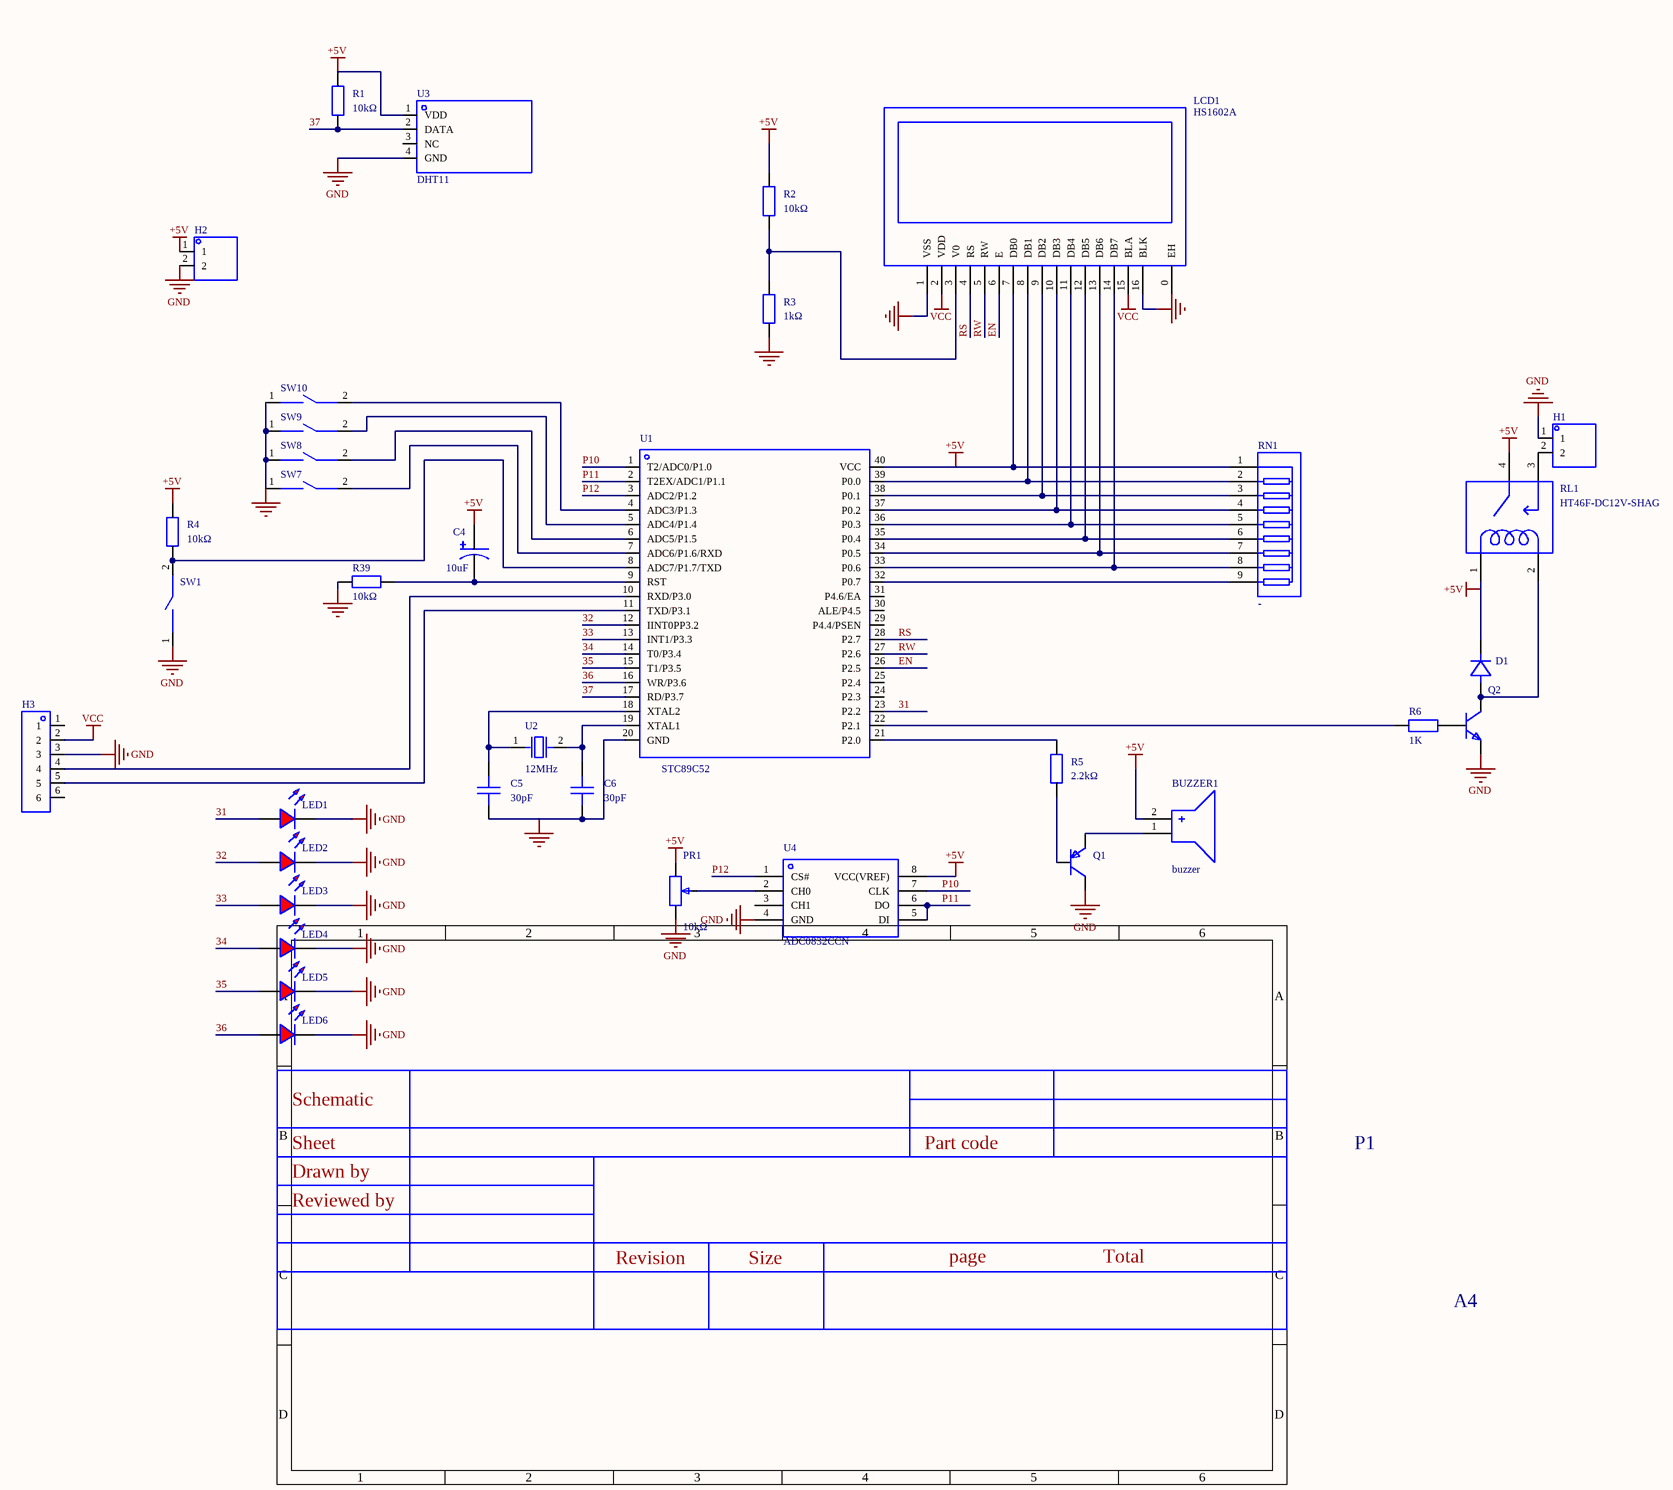
[diagram p0: MISC89128-3.schdoc]
# Altium project MISC89128-2.PrjPcb
1 sheet, 36 parts. Net scope: global (net labels, ports and power ports of the same name join across sheets).
Board file: MISC89128.pcbdoc

## Sheet MISC89128-3.schdoc
size 178 x 98 mm; Version: V1.0; @Project Name: MISC89128; @Page Count: 1; @Update Date: 2026-04-20; @Create Date: 2026-04-20; @Schematic Name: MISC89128; @Page No: 1; @Board Name: MISC89128; @Create Time: 15:46:19; @Update Time: 15:42:54

### Parts
BUZZER1  buzzer  [BUZ-TH_BD12.0-P6.00-D0.9-RD]
C4  10uF  [CAP-TH_BD6.3-P2.50-D1.0-FD]
C5  30pF  [CAP-TH_L3.6-W2.3-P5.00-D0.5]
C6  30pF  [CAP-TH_L3.6-W2.3-P5.00-D0.5]
D1  (no value)  [DO_1N4007]
H1  (no value)  [HDR-TH_2P-P2.54-V-M-1]
H2  (no value)  [HDR-TH_2P-P2.54-V-M-1]
H3  (no value)  [HDR-TH_6P-P2.54-V-F]
LCD1  HS1602A  [LCD1602]
LED1  (no value)  [LED_TH-3mm]
LED2  (no value)  [LED_TH-3mm]
LED3  (no value)  [LED_TH-3mm]
LED4  (no value)  [LED_TH-3mm]
LED5  (no value)  [LED_TH-3mm]
LED6  (no value)  [LED_TH-3mm]
PR1  10kΩ  [R_3296]
Q1  (no value)  [S8550P_SOT]
Q2  (no value)  [S8050_SOT-23]
R1  10kΩ  [Res_1/8W]
R2  10kΩ  [Res_1/8W]
R3  1kΩ  [Res_1/8W]
R4  10kΩ  [Res_1/8W]
R5  2.2kΩ  [Res_1/8W]
R6  1K  [R0805]
R39  10kΩ  [Res_1/8W]
RL1  HT46F-DC12V-SHAG  [RELAY-TH_HT46F-DCXXV-SHAG]
RN1  -  [RES-ARRAY-TH_9P-P2.54-D1.0]
SW1  Tact switch, 6*6*5 plastic head, 260G, travel 0.25mm, through-hole 2-pin  [KEY-TH_2P-L6.0-W6.0-P5.00]  (value not drawn)
SW7  Tact switch, 6*6*5 plastic head, 260G, travel 0.25mm, through-hole 2-pin  [KEY-TH_2P-L6.0-W6.0-P5.00]  (value not drawn)
SW8  Tact switch, 6*6*5 plastic head, 260G, travel 0.25mm, through-hole 2-pin  [KEY-TH_2P-L6.0-W6.0-P5.00]  (value not drawn)
SW9  Tact switch, 6*6*5 plastic head, 260G, travel 0.25mm, through-hole 2-pin  [KEY-TH_2P-L6.0-W6.0-P5.00]  (value not drawn)
SW10  Tact switch, 6*6*5 plastic head, 260G, travel 0.25mm, through-hole 2-pin  [KEY-TH_2P-L6.0-W6.0-P5.00]  (value not drawn)
U1  STC89C52  [DIP-40_L52.3-W13.9-P2.54-LS15.2-BL]
U2  12MHz  [HC-49US_L11.0-W4.6-P4.88]
U3  DHT11  [SENSOR-TH_DHT11]
U4  ADC0832CCN  [DIP-8_L9.7-W6.4-P2.54-LS7.6-BL]

### Nets
+5V: BUZZER1.2(+) C4.1 D1.1(K) H2.1 LCD1.7(DB0) PR1.3 R1.2 R2.2 R4.2 RL1.1 RL1.4 RN1.1 U1.40(VCC) U3.1(VDD) U4.8(VCC(VREF))
GND: C5.1 C6.1 H1.1 H2.2 H3.3 LCD1.1(VSS) LCD1.16(BLK) LED1.2(A) LED2.2(A) LED3.2(A) LED4.2(A) LED5.2(A) LED6.2(A) PR1.1 Q1.3(C) Q2.2 R3.1 R39.1 SW1.1 SW7.1 SW8.1 SW9.1 SW10.1 U1.20(GND) U3.4(GND) U4.4(GND)
VCC: H3.2 LCD1.2(VDD) LCD1.15(BLA)
31: LED1.1(C) U1.23(P2.2)
32: LED2.1(C) U1.12(IINT0PP3.2)
33: LED3.1(C) U1.13(INT1/P3.3)
34: LED4.1(C) U1.14(T0/P3.4)
35: LED5.1(C) U1.15(T1/P3.5)
36: LED6.1(C) U1.16(WR/P3.6)
37: R1.1 U1.17(RD/P3.7) U3.2(DATA)
EN: LCD1.6(E) U1.26(P2.5)
P10: U1.1(T2/ADC0/P1.0) U4.7(CLK)
P11: U1.2(T2EX/ADC1/P1.1) U4.5(DI) U4.6(DO)
P12: U1.3(ADC2/P1.2) U4.1(CS#)
RS: LCD1.4(RS) U1.28(P2.7)
RW: LCD1.5(RW) U1.27(P2.6)
NetBUZZER1_1: BUZZER1.1(-) Q1.2(E)
NetC4_2: C4.2 R39.2 U1.9(RST)
NetC5_2: C5.2 U1.18(XTAL2) U2.1(OSC1)
NetC6_2: C6.2 U1.19(XTAL1) U2.2(OSC2)
NetD1_2: D1.2(A) Q2.3 RL1.2
NetH1_2: H1.2 RL1.3
NetH3_4: H3.4 U1.10(RXD/P3.0)
NetH3_5: H3.5 U1.11(TXD/P3.1)
NetLCD1_3: LCD1.3(V0) R2.1 R3.2
NetLCD1_8: LCD1.8(DB1) RN1.2 U1.39(P0.0)
NetLCD1_9: LCD1.9(DB2) RN1.3 U1.38(P0.1)
NetLCD1_10: LCD1.10(DB3) RN1.4 U1.37(P0.2)
NetLCD1_11: LCD1.11(DB4) RN1.5 U1.36(P0.3)
NetLCD1_12: LCD1.12(DB5) RN1.6 U1.35(P0.4)
NetLCD1_13: LCD1.13(DB6) RN1.7 U1.34(P0.5)
NetLCD1_14: LCD1.14(DB7) RN1.8 U1.33(P0.6)
NetPR1_2: PR1.2 U4.2(CH0)
NetQ1_1: Q1.1(B) R5.1
NetQ2_1: Q2.1 R6.1
NetR4_1: R4.1 SW1.2 U1.8(ADC7/P1.7/TXD)
NetR5_2: R5.2 U1.21(P2.0)
NetR6_2: R6.2 U1.22(P2.1)
NetRN1_9: RN1.9 U1.32(P0.7)
NetSW7_2: SW7.2 U1.7(ADC6/P1.6/RXD)
NetSW8_2: SW8.2 U1.6(ADC5/P1.5)
NetSW9_2: SW9.2 U1.5(ADC4/P1.4)
NetSW10_2: SW10.2 U1.4(ADC3/P1.3)

Not connected (* = marked no-connect by the designer): H3 1 6; LCD1 0(EH); U1 24(P2.3) 25(P2.4) 29(P4.4/PSEN) 30(ALE/P4.5) 31(P4.6/EA); U3 3(NC); U4 3(CH1)

### Notes on the sheet
- 2026-04-20
- Schematic
- Sheet
- Part code
- P1
- Reviewed by
- Drawn by
- Revision
- Size
- page
- Total
- A4
- 1

### Library data of the parts
BUZZER1 = buzzer: AddInBom: yes; ModelId: af17e4151ed84fc2a628230bf23763630819f05c4eef4c71ace90d822a990e87; ModelTransform: 472.44,472.176,0,270,0,0,0,0,-196.85; Symbol: BUZZER; Device: buzzer; LCSC Part Name: buzzer; SupplierPart: C9900014030; ManufacturerPart: buzzer; Supplier Footprint: buzzer; JLCPCB Part Class: Extended Part; Supplier: LCSC; ConvertToPcb: yes; FootprintName: BUZ-TH_BD12.0-P6.00-D0.9-RD; ModelName: BUZ-TH_BD12.0-P6.00-D0.9-RD
C4 = LKMC1202E100MF: Capacitance: 10uF; tolerance: ±20%; rated voltage: 250V; ripple current: -; equivalent series resistance: -;; Manufacturer: Ymin(永铭); AddInBom: yes; ModelId: 0a4db4bf24b443b3be4905be97ff10c5; ModelTransform: 248.4247,247.99777,0,0,0,0,0,0,-137.795; φD: 6.3mm; L: 12mm; Lifetime @ Temp: 9000hrs@105℃; Symbol: LKMC1202E100MF; Device: LKMC1202E100MF; LCSC Part Name: 10uF ±20% 250V; SupplierPart: C443243; ManufacturerPart: LKMC1202E100MF; Supplier Footprint: 插件,D6.3xL12mm; JLCPCB Part Class: Extended library; Datasheet: example.com/20200220/C487520_443A40905984A455D375EE990FEAA9E8.pdf; Supplier: LCSC; ConvertToPcb: yes; FootprintName: CAP-TH_BD6.3-P2.50-D1.0-FD; ModelName: CAP-TH_BD6.3-P2.50-D1.0-FD; Value: 10uF; Tolerance: ±20%; Rated Voltage: 250V; Ripple Current: -; Equivalent Series Resistance(ESR): -; Lead Spacing: 2.5mm
C5 C6 = K300J10C0GF5UH5: Capacitance: 30pF; tolerance: ±5%; rated voltage: 50V; temperature coefficient: C0G;; Manufacturer: VISHAY(威世); AddInBom: yes; ModelId: 8586b865f3f94c6bbd5d7f2c3c951380; ModelName: CAP-TH-2P-L3.6-W2.3-H6.2-P5.0; ModelTransform: 220.472,90.551,0,0,0,0,-0.005,0,-137.795; Symbol: K300J10C0GF5UH5; Device: K300J10C0GF5UH5; LCSC Part Name: 30pF ±5% 50V; SupplierPart: C1623919; ManufacturerPart: K300J10C0GF5UH5; Supplier Footprint: 插件; JLCPCB Part Class: Extended library; Datasheet: example.com/20210702/6531D680143ED60327F22057485455BA.pdf; Supplier: LCSC; ConvertToPcb: yes; FootprintName: CAP-TH_L3.6-W2.3-P5.00-D0.5; Value: 30pF; Tolerance: ±5%; Voltage Rated: 50V; Temperature Coefficient: C0G
D1 = D_1N4007A: AddInBom: yes; ModelId: 6de1e9b71a0d4751b4e9df530304c1a30819f05c4eef4c71ace90d822a990e87; ModelName: DO-41_D2.4-L4.7-P8.70; ModelTransform: 373.9,94.4,232.29,0,0,0,0,0,-140; Symbol: D_1N4007; Device: D_1N4007A; Supplier Footprint: DO-41; ConvertToPcb: yes; FootprintName: DO_1N4007
H1 H2 = HDR-M_2.54_1x2P: Symbol: 210S-1*2P L=11.6MMGold-plated black; ConvertToPcb: yes; ModelId: 79b2e9f2d70a4d68a1b7098f27c6d4c5; ModelName: HDR-M-2.54_1x2; ModelTransform: 200,100,0,0,0,0,0,0,-118.11; Device: HDR-M_2.54_1x2P; AddInBom: yes; SupplierPart: C124375; Supplier Footprint: 插件; FootprintName: HDR-TH_2P-P2.54-V-M-1
H3 = HDR-F_2.54_1x6P: Symbol: Header-Female-2.54_1x6; ConvertToPcb: yes; ModelId: 0f5bcf94dcda47d085f24cdca1696fe90819f05c4eef4c71ace90d822a990e87; ModelTransform: 619.684,94.488,0,0,0,0,0,0,-125.984; Device: HDR-F_2.54_1x6P; AddInBom: yes; SupplierPart: C40877; Supplier Footprint: 插件; FootprintName: HDR-TH_6P-P2.54-V-F; ModelName: HDR-TH_6P-P2.54-V-F
LCD1 = HS1602A: Main control chip: SPLC780; size (inch): 2;; Manufacturer: HS(汉昇); AddInBom: yes; ModelId: f9d832f46a914cadb50fc4d4cefd25170819f05c4eef4c71ace90d822a990e87; ModelTransform: 3149.6,1417.32,0,0,0,0,0,0,-118.11; Symbol: HS1602A; Device: HS1602A; LCSC Part Name: 2.0寸16*2单色字符字符液晶显示屏; SupplierPart: C5329588; ManufacturerPart: HS1602A; Supplier Footprint: -; JLCPCB Part Class: Extended Part; Datasheet: example.com/20221212/35734F14DBB323F90DD8DBE1717CD9FD.pdf; Supplier: LCSC; ConvertToPcb: yes; FootprintName: LCD1602; ModelName: LCD1602; Main Control Chip: SPLC780; Size: 2; Operating Temperature: -20℃~+70℃
LED1-LED6 = LED_TH-R_3mm: ConvertToPcb: yes; ModelId: a497c992633541038a38947cdc58012f0819f05c4eef4c71ace90d822a990e87; ModelName: LED-TH-3mm_R; ModelTransform: 141.274,153.327,0,0,0,0,-5.984,0,-137.795; Symbol: LED_TH-R; Device: LED_TH-R_3mm; AddInBom: yes; FootprintName: LED_TH-3mm; Supplier Footprint: 插件
PR1 = R_3296: ConvertToPcb: yes; ModelId: b182808559bb43bda9e7de64b64134cb0819f05c4eef4c71ace90d822a990e87; ModelName: 3296W; ModelTransform: 373.98,188.96,590.49,180,0,0,0,0,-140; Symbol: R_3296; Device: R_3296; AddInBom: yes; Supplier Footprint: 直插; FootprintName: R_3296; Value: 10kΩ
Q1 = S8550_SOT_PNP: Symbol: PNP; ConvertToPcb: yes; ModelId: 9c0df02d6f3e44e889da37f3e5bf54960819f05c4eef4c71ace90d822a990e87; ModelName: SOT-23-3_L2.9-W1.4-P1.90-LS2.5-BR; ModelTransform: 98.43,114.17,37.91,0,0,0,0,0,0; Device: S8550_SOT_PNP; AddInBom: yes; Supplier Footprint: SOT-23; FootprintName: S8550P_SOT
Q2 = S8050_SOT_NPN: Symbol: NPN; ConvertToPcb: yes; ModelId: c62791f0466c4ae2a892c056b845b0ca0819f05c4eef4c71ace90d822a990e87; ModelName: SOT-23-3P_L2.9-W1.3-H1.0-LS2.4-P0.95; ModelTransform: 98.6,114.12,41.29,180,0,0,0,0,-3; Device: S8050_SOT_NPN; AddInBom: yes; Supplier Footprint: SOT-23; FootprintName: S8050_SOT-23
R1-R5 = Res_AXIAL-1/8W: Symbol: Resistor; 3D Model: b2b5ae7ae4c642178fe0039925c86a3f; 3D Model Transform: 282.86,66.88,253.09,0,0,0,0,0,-191; ConvertToPcb: yes; ModelName: RES-TH_BD1.8-L3.2-P7.20-D0.4; Device: Res_AXIAL-1/8W; Supplier Footprint: 轴向引线; AddInBom: yes; FootprintName: Res_1/8W
  R1 R2 R4: Value: 10kΩ
  R3: Value: 1kΩ
  R5: Value: 2.2kΩ
R6 = Res_0805: Symbol: Resistor; 3D Model: 37a81e68749a4138bd2dfa6897b24b85; 3D Model Transform: 78.74,51.181,0,0,0,0,0,-0.0005,0; ConvertToPcb: yes; ModelName: R0805_L2.0-W1.3-H0.6; Device: Res_0805; Value: 1K; Supplier Footprint: 0805; AddInBom: yes; FootprintName: R0805
R39 = Res_AXIAL-1/8W: Symbol: Resistor; ConvertToPcb: yes; ModelId: b2b5ae7ae4c642178fe0039925c86a3f; ModelName: RES-TH_BD1.8-L3.2-P7.20-D0.4; ModelTransform: 282.86,66.88,253.09,0,0,0,0,0,-191; Device: Res_AXIAL-1/8W; AddInBom: yes; Supplier Footprint: 轴向引线; Value: 10kΩ; FootprintName: Res_1/8W
RL1 = HT46F-DC12V-SHAG: AddInBom: yes; ModelId: 502250c4816b48b39cafff0c843eaac20819f05c4eef4c71ace90d822a990e87; ModelTransform: 826.77,279.9207,0,0,0,0,3.937,0,-137.795; Symbol: HT46F-DC12V-SHAG; Device: HT46F-DC12V-SHAG; LCSC Part Name: HT46F-DC12V-SHAG; SupplierPart: C9900113369; ManufacturerPart: HT46F-DC12V-SHAG; Supplier Footprint: 继电器; Supplier: LCSC; ConvertToPcb: yes; FootprintName: RELAY-TH_HT46F-DCXXV-SHAG; ModelName: RELAY-TH_HT46F-DCXXV-SHAG
RN1 = 排阻 10 K 5%: Number of resistors: -; resistance: -; power per element: -;; Symbol: 10 K 5%; Device: Resistor array 10 K 5%; AddInBom: yes; ModelId: d106c67f29e14d8080ba548247a719a10819f05c4eef4c71ace90d822a990e87; ModelName: SIP-9_L22.8-W3.0-H8.5-P2.54; ModelTransform: 918.1084,118.11,0,0,0,0,0,0,-137.795; LCSC Part Name: 10KΩ (103) ±5%; SupplierPart: C26615; ManufacturerPart: 排阻 10 K 5%; Supplier Footprint: 插件; JLCPCB Part Class: Extended Part; Supplier: LCSC; ConvertToPcb: yes; FootprintName: RES-ARRAY-TH_9P-P2.54-D1.0; Number of Resistors: -; Value: -; Power(Watts): -; Number of Pins: -
SW1 SW7-SW10 = 轻触开关,6*6*5塑头,260G,行程0.25mm,直插中2脚: Symbol: SWITCH,6*6*5PLASTIC HEAD,260G, 0.25MM,DIP2; 3D Model: d13ad252cbf84dc495704a853cd2bab6; 3D Model Transform: 236.22,236.22,0,0,0,0,0,0,-137.795; AddInBom: yes; ModelName: KEY-TH_2P-L6.0-W6.0-H5.0-P5.00; Device: Tact switch, 6*6*5 plastic head, 260G, travel 0.25mm, through-hole 2-pin; LCSC Part Name: 轻触开关,6*6*5塑头,260G,行程0.25mm,直插中2脚; Supplier Part: C71845; Manufacturer Part: 轻触开关,6*6*5塑头,260G,行程0.25mm,直插中2脚; Supplier Footprint: 插件; JLCPCB Part Class: Extended library; Supplier: LCSC; ConvertToPcb: yes; FootprintName: KEY-TH_2P-L6.0-W6.0-P5.00
U1 = STC89C516RD+40I-PDIP40: CPU core: 51 series; program storage: 61KB; total RAM: 1.25KB; GPIO port count: 35; operating voltage: 3.5V~5.5V; CPU max frequency: -; program memory type: FLASH;; Manufacturer: STC(宏晶); AddInBom: yes; ModelId: 16d4686a009b4ddca948f91eddb57b14; ModelName: DIP-40_L52.3-W13.8-H4.0-LS15.24-P2.54; ModelTransform: 2059.051,615.743,0,0,0,0,0,0,-129.921; GPIO Ports Number: 35; 16Bit Timer: 3; UART/USART: 1; Peripheral/Function: Watchdog; Symbol: STC89C516RD+40I-PDIP40; Device: STC89C516RD+40I-PDIP40; Manufacturer Part: STC89C52; LCSC Part Name: STC89C516RD+40I-PDIP40; SupplierPart: C52225; Supplier Footprint: DIP-40; JLCPCB Part Class: Extended library; Datasheet: example.com/20180614/C87831_BBAF7FB8B286C29ACE4E9B180C033FEC.pdf; Supplier: LCSC; ConvertToPcb: yes; FootprintName: DIP-40_L52.3-W13.9-P2.54-LS15.2-BL; CPU Core: 51 series; Program Storage Size: 61KB; RAM Size: 1.25KB; Operating Voltage Range: 3.5V~5.5V; CPU Maximum Speed: -; Program Memory Type: FLASH; Operating Temperature Range: -40℃~+85℃; ADC (Bit): -; DAC (Bit): -; PWM (Bit): -; 8Bit Timer: -; 32Bit Timer: -; CAN: -; I2C: -; I2S: -; SPI: -; Universal Serial Bus: -; Internal Comparator: -; communication protocol: -; Watchdog: Yes; Real-Time Clock: -; Infrared Data Association: -; Low-Voltage Detect: -; CCP Capture/Compare: -; Secure Digital Input and Output: -; Direct Memory Access: -; Internal Oscillator: -
U2 = ECS-120-S-4: Frequency: 12MHz; room-temperature frequency tolerance: ±30ppm; external load capacitance: -; frequency stability (full temperature): ±50ppm;; Manufacturer: ECS; AddInBom: yes; ModelId: 59d05c800eee432cb051aa4925461fda; ModelName: HC-49US_L11.0-W4.7-H3.5-P4.88; ModelTransform: 432.44473,183.0705,0,0,0,0,0,0,-137.795; Equivalent Series Resistance (ESR): 60Ω; Symbol: ECS-120-S-4; Device: ECS-120-S-4; LCSC Part Name: 12MHz ±30ppm; ManufacturerPart: ECS-120-S-4; Supplier Footprint: HC-49S; JLCPCB Part Class: Extended library; Datasheet: example.com/20210402/81F084B668D60DFAE850A61100CCABAF.pdf; Supplier: LCSC; ConvertToPcb: yes; FootprintName: HC-49US_L11.0-W4.6-P4.88; Value: 12MHz; Normal temperature Frequency Tolerance: ±30ppm; External load capacitor: -; Frequency Stability(Full temperature range): ±50ppm; Operating Temperature: -10℃~+70℃
U3 = DHT11: New capacitive digital temperature and humidity sensor; old model discontinued, 16.1x12.6x5.8mm; Manufacturer: 广州奥松; 3D Model: 6dde47d4d8bf4fa598dffcc067449c1d; 3D Model Transform: 236.25937,492.125,0,270,0,0,0,-11.811,-196.85; AddInBom: yes; Symbol: DHT11; Device: DHT11; LCSC Part Name: DHT11  电容式传感器 新款电容式数字温湿度传感器,老款已停产16.1x12.6x5.8mm; Supplier Part: C117051; Manufacturer Part: DHT11; Supplier Footprint: SIP-4; JLCPCB Part Class: Extended library; Datasheet: example.com/20170703/1499081238365.pdf; Supplier: LCSC; ConvertToPcb: yes; FootprintName: SENSOR-TH_DHT11; ModelName: SENSOR-TH_DHT11
U4 = ADC0832CCN: AddInBom: yes; ModelId: 5746b540d01a4d1b9eb6b4f989297bc70819f05c4eef4c71ace90d822a990e87; ModelName: DIP-8_L9.8-W6.6-H3.5-LS7.62-P2.54; ModelTransform: 385.826,311.8104,0,0,0,0,0,0,-118.11; Symbol: ADC0832CCN; Device: ADC0832CCN; LCSC Part Name: ADC0832CCN; SupplierPart: C10915; ManufacturerPart: ADC0832CCN; Supplier Footprint: DIP-8; JLCPCB Part Class: Extended Part; Supplier: LCSC; ConvertToPcb: yes; FootprintName: DIP-8_L9.7-W6.4-P2.54-LS7.6-BL